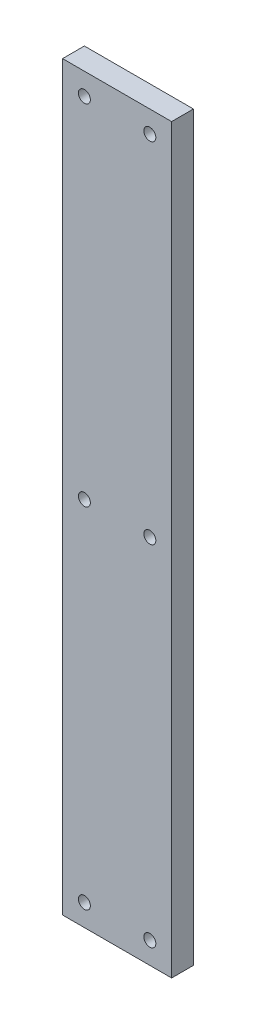
from build123d import *

# Parameters (mm, degrees)
SKETCH1_W            = 100
SKETCH1_H            = 680
BOSS_EXTRUDE1_DEPTH  = 20
SKETCH2_R            = 5.5
CUT_EXTRUDE1_DEPTH   = 20
LPATTERN1_COUNT      = 2
LPATTERN1_PITCH      = 60
LPATTERN1_COUNT_DIR2 = 3
LPATTERN1_PITCH_DIR2 = 320


with BuildPart() as part:
    # Sketch1 → Boss-Extrude1 (new body)
    with BuildSketch(Plane.XY):
        with Locations((50, -340)):
            Rectangle(SKETCH1_W, SKETCH1_H)
    extrude(amount=BOSS_EXTRUDE1_DEPTH)

    # Sketch2 → Cut-Extrude1 (cut)
    with BuildSketch(Plane.XY.offset(20)):
        with Locations((20, -20)):
            Circle(SKETCH2_R)
    cut_extrude1 = extrude(amount=-CUT_EXTRUDE1_DEPTH, mode=Mode.SUBTRACT)

    # LPattern1: Cut-Extrude1 2 × 3
    with Locations(*[(i * LPATTERN1_PITCH, -j * LPATTERN1_PITCH_DIR2, 0) for i in range(LPATTERN1_COUNT) for j in range(LPATTERN1_COUNT_DIR2) if (i, j) != (0, 0)]):
        add(cut_extrude1, mode=Mode.SUBTRACT)


solid = part.part
